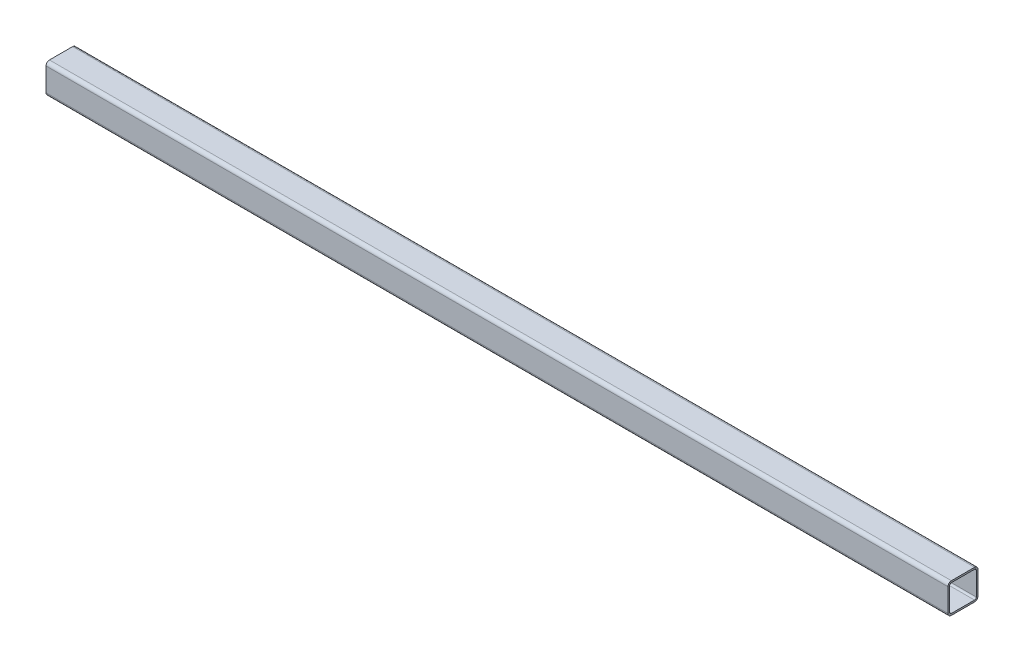
from build123d import *

# Parameters (mm, degrees)
SQUARE_TUBE_40_X_40_X_2_3_1_DEPTH = 1200


with BuildPart() as part:
    # Sketch11 → Square Tube 40 X 40 X 2.3(1) (new body)
    with BuildSketch(Plane.YZ):
        with BuildLine():
            Line((-15.4, -20), (15.4, -20))
            ThreePointArc((15.4, -20), (18.652691193, -18.652691193), (20, -15.4))
            Line((20, -15.4), (20, 15.4))
            ThreePointArc((20, 15.4), (18.652691193, 18.652691193), (15.4, 20))
            Line((15.4, 20), (-15.4, 20))
            ThreePointArc((-15.4, 20), (-18.652691193, 18.652691193), (-20, 15.4))
            Line((-20, 15.4), (-20, -15.4))
            ThreePointArc((-20, -15.4), (-18.652691193, -18.652691193), (-15.4, -20))
        make_face()
        with BuildLine():
            Line((-15.4, -17.7), (15.4, -17.7))
            ThreePointArc((15.4, -17.7), (17.026345597, -17.026345597), (17.7, -15.4))
            Line((17.7, -15.4), (17.7, 15.4))
            ThreePointArc((17.7, 15.4), (17.026345597, 17.026345597), (15.4, 17.7))
            Line((15.4, 17.7), (-15.4, 17.7))
            ThreePointArc((-15.4, 17.7), (-17.026345597, 17.026345597), (-17.7, 15.4))
            Line((-17.7, 15.4), (-17.7, -15.4))
            ThreePointArc((-17.7, -15.4), (-17.026345597, -17.026345597), (-15.4, -17.7))
        make_face(mode=Mode.SUBTRACT)
    extrude(amount=SQUARE_TUBE_40_X_40_X_2_3_1_DEPTH)


solid = part.part
